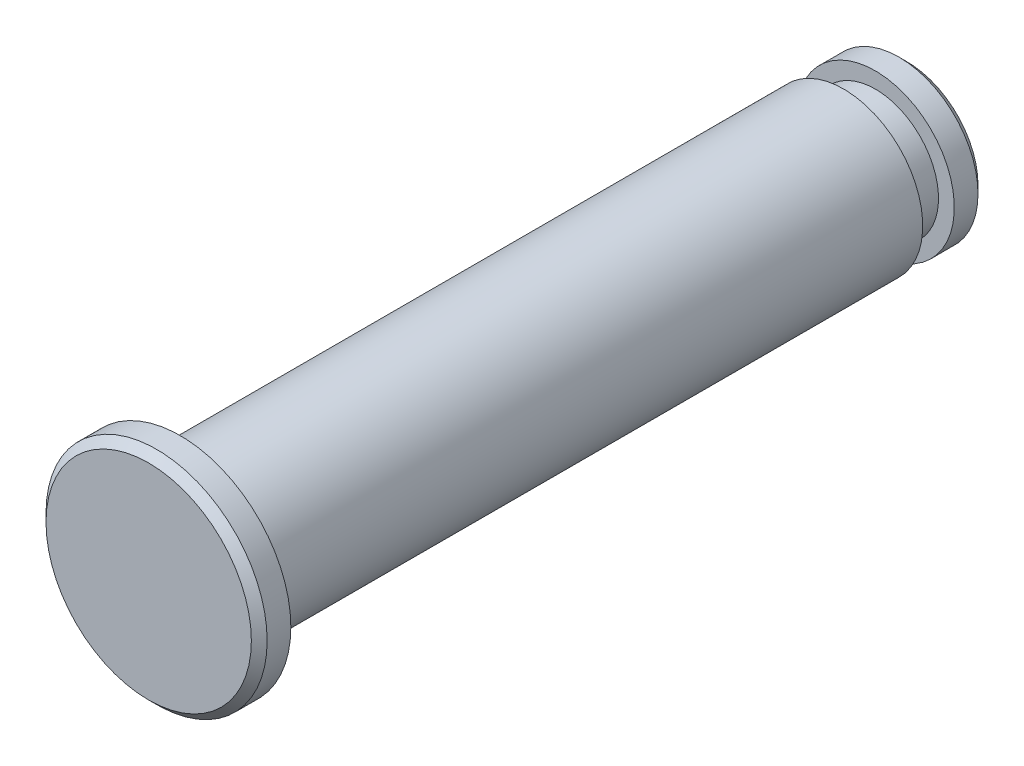
from build123d import *

# Parameters (mm, degrees)
SKETCH1_R               = 5
BOSS_EXTRUDE1_DEPTH     = 46
SKETCH2_R               = 7
BOSS_EXTRUDE2_DEPTH     = 2
CHAMFER1_SIZE           = 0.5
SKETCH3_R               = 14
SKETCH3_R_2             = 4
CUT_EXTRUDE_THIN1_DEPTH = 2


with BuildPart() as part:
    # Sketch1 → Boss-Extrude1 (new body)
    with BuildSketch(Plane.XY):
        Circle(SKETCH1_R)
    extrude(amount=BOSS_EXTRUDE1_DEPTH)

    # Sketch2 → Boss-Extrude2 (add)
    with BuildSketch(Plane.XY.offset(46)):
        Circle(SKETCH2_R)
    extrude(amount=BOSS_EXTRUDE2_DEPTH)

    # Chamfer1
    chamfer1_edges = [part.edges().sort_by_distance(p)[0] for p in [
        (-5, 0, 0),
        (-7, 0, 48),
    ]]
    chamfer(chamfer1_edges, length=CHAMFER1_SIZE)

    # Sketch3 → Cut-Extrude-Thin1 (cut)
    with BuildSketch(Plane(origin=(0, 0, 2), x_dir=(-1, 0, 0), z_dir=(0, 0, -1))):
        Circle(SKETCH3_R)
        Circle(SKETCH3_R_2, mode=Mode.SUBTRACT)
    extrude(amount=-CUT_EXTRUDE_THIN1_DEPTH, mode=Mode.SUBTRACT)


solid = part.part
